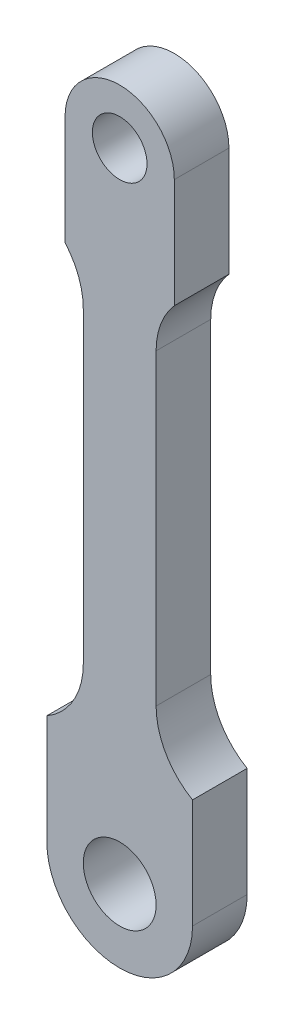
from build123d import *

# Parameters (mm, degrees)
SKETCH1_R           = 1.5
SKETCH1_R_2         = 2
BOSS_EXTRUDE1_DEPTH = 1.5


with BuildPart() as part:
    # Sketch1 → Boss-Extrude1 (new, symmetric)
    with BuildSketch(Plane.XY):
        with BuildLine():
            Line((-3, 0), (-3, -6))
            ThreePointArc((-3, -6), (-2.258342613, -7.231537749), (-2, -8.645751311))
            Line((-2, -8.645751311), (-2, -25.535898385))
            ThreePointArc((-2, -25.535898385), (-2.535898385, -27.535898385), (-4, -29))
            Line((-4, -29), (-4, -35))
            ThreePointArc((-4, -35), (0, -39), (4, -35))
            Line((4, -35), (4, -29))
            ThreePointArc((4, -29), (2.535898385, -27.535898385), (2, -25.535898385))
            Line((2, -25.535898385), (2, -8.645751311))
            ThreePointArc((2, -8.645751311), (2.258342613, -7.231537749), (3, -6))
            Line((3, -6), (3, 0))
            ThreePointArc((3, 0), (0, 3), (-3, 0))
        make_face()
        Circle(SKETCH1_R, mode=Mode.SUBTRACT)
        with Locations((0, -35)):
            Circle(SKETCH1_R_2, mode=Mode.SUBTRACT)
    extrude(amount=BOSS_EXTRUDE1_DEPTH, both=True)


solid = part.part
